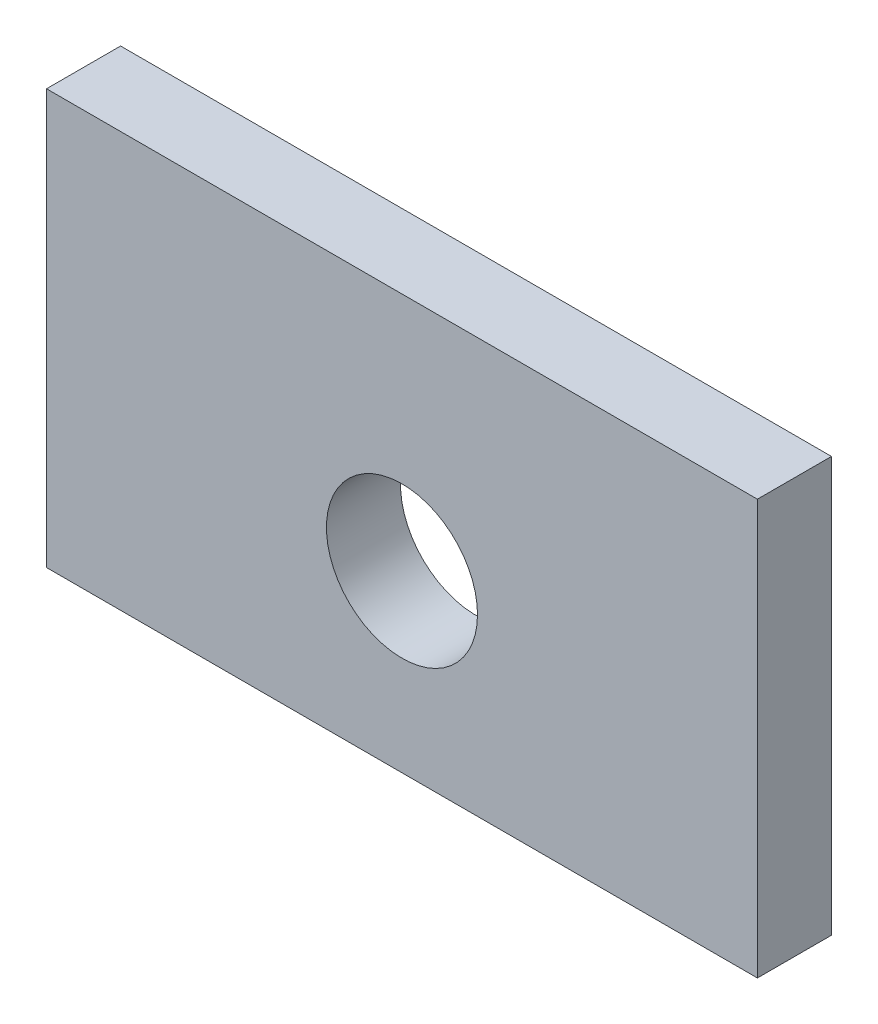
SolidWorks part; units mm, degrees
material "Q235"
ref_plane "Front Plane" through (0, 0, 0) normal (0, 0, 1) x (1, 0, 0)
ref_plane "Top Plane" through (0, 0, 0) normal (0, 1, 0) x (1, 0, 0)
ref_plane "Right Plane" through (0, 0, 0) normal (1, 0, 0) x (0, 0, -1)
sketch "Sketch1" plane through (0, 0, 0) normal (0, 0, 1) x (1, 0, 0)
  line L1 (0, 0) -> (240, 0)
  line L2 (0, 0) -> (0, 140)
  line L3 (0, 140) -> (240, 140)
  line L4 (240, 0) -> (240, 140)
  circle A0 centre (120, 59) radius 25.5
  dimension "D3" = 51
  dimension "D4" = 120
  dimension "D5" = 59
  dimension "D1" = 240
  dimension "D2" = 140
extrude "Boss-Extrude1" add sketch "Sketch1" along normal blind 25
